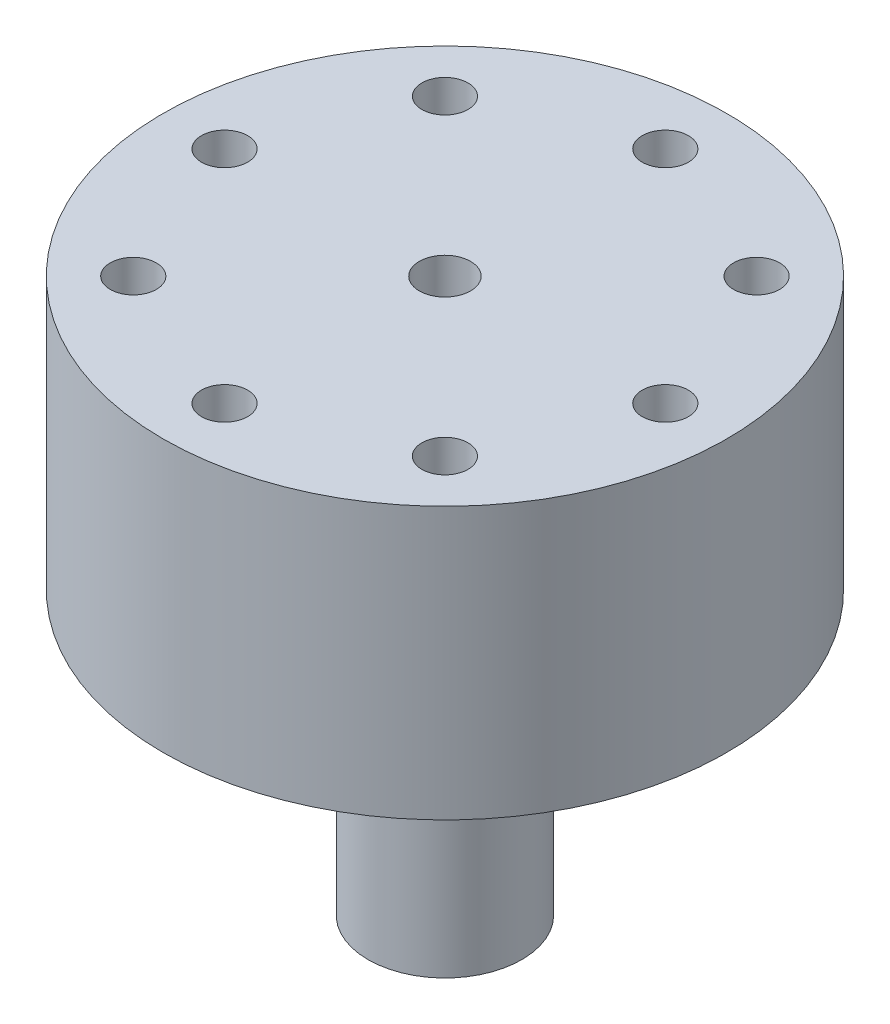
SolidWorks part; units mm, degrees
ref_plane "前视基准面" through (0, 0, 0) normal (0, 0, 1) x (1, 0, 0)
ref_plane "上视基准面" through (0, 0, 0) normal (0, 1, 0) x (1, 0, 0)
ref_plane "右视基准面" through (0, 0, 0) normal (1, 0, 0) x (0, 0, -1)
sketch "草图1" plane through (0, 0, 0) normal (0, 0, 1) x (1, 0, 0)
  line L0 (0, 13.8883) -> (0, -13.9905) construction
  line L1 (5, 13.2235) -> (5, 0.2651)
  line L2 (24.2332, -39.7765) -> (55, -39.7765)
  line L3 (55, -39.7765) -> (55, 13.2235)
  line L4 (55, 13.2235) -> (5, 13.2235)
  line L5 (0, -13.9905) -> (0, -46.4659) construction
  arc A0 (24.2332, -39.7765) -> (5, 0.2651) centre (0, -26.7765) ccw
  dimension "D4" = 55
  dimension "D5" = 40
  dimension "D1" = 5
  dimension "D2" = 50
  dimension "D3" = 53
revolve "旋转1" add sketch "草图1" angle 360 about L0
sketch "草图2" plane through (0, -39.7765, 0) normal (0, -1, 0) x (1, 0, 0)
  circle A0 centre (43, 0) radius 7.5
  circle A1 centre (0, 0) radius 5 construction
  circle A2 centre (30.4056, -30.4056) radius 7.5
  circle A3 centre (0, -43) radius 7.5
  circle A4 centre (-30.4056, -30.4056) radius 7.5
  circle A5 centre (-43, 0) radius 7.5
  circle A6 centre (-30.4056, 30.4056) radius 7.5
  circle A7 centre (0, 43) radius 7.5
  circle A8 centre (30.4056, 30.4056) radius 7.5
  point P20 (0, 0)
  dimension "D1" = 15
  dimension "D2" = 43
  dimension "D3" = 8
extrude "切除-拉伸1" cut sketch "草图2" against normal blind 2
sketch "草图5" plane through (0, -37.7765, 0) normal (0, -1, 0) x (1, 0, 0)
  circle A0 centre (0, 43) radius 4.5
  circle A1 centre (30.4056, 30.4056) radius 4.5
  circle A2 centre (43, 0) radius 4.5
  circle A3 centre (30.4056, -30.4056) radius 4.5
  circle A4 centre (0, -43) radius 4.5
  circle A5 centre (-30.4056, -30.4056) radius 4.5
  circle A6 centre (-43, 0) radius 4.5
  circle A7 centre (-30.4056, 30.4056) radius 4.5
  point P19 (0, 0)
  dimension "D1" = 9
  dimension "D2" = 8
extrude "切除-拉伸2" cut sketch "草图5" against normal up to next
sketch "草图7" plane through (0, -39.7765, 0) normal (0, -1, 0) x (1, 0, 0)
  circle A0 centre (0, 0) radius 30.7216
  dimension "D1" = 61.4432
extrude "凸台-拉伸1" add sketch "草图7" against normal blind 41
sketch "草图8" plane through (0, -39.7765, 0) normal (0, -1, 0) x (1, 0, 0)
  circle A0 centre (0, 0) radius 17.5
  dimension "D1" = 35
extrude "凸台-拉伸2" add sketch "草图8" along normal blind 10
sketch "草图9" plane through (0, -49.7765, 0) normal (0, -1, 0) x (1, 0, 0)
  circle A0 centre (0, 0) radius 15
  dimension "D1" = 30
extrude "凸台-拉伸3" add sketch "草图9" along normal blind 45
sketch "草图10" plane through (0, -49.7765, 0) normal (0, -1, 0) x (1, 0, 0)
  circle A0 centre (0, 0) radius 15 construction
  circle A1 centre (0, 0) radius 15
  circle A2 centre (0, 0) radius 13
  dimension "D1" = 26
extrude "切除-拉伸3" cut sketch "草图10" along normal blind 2
